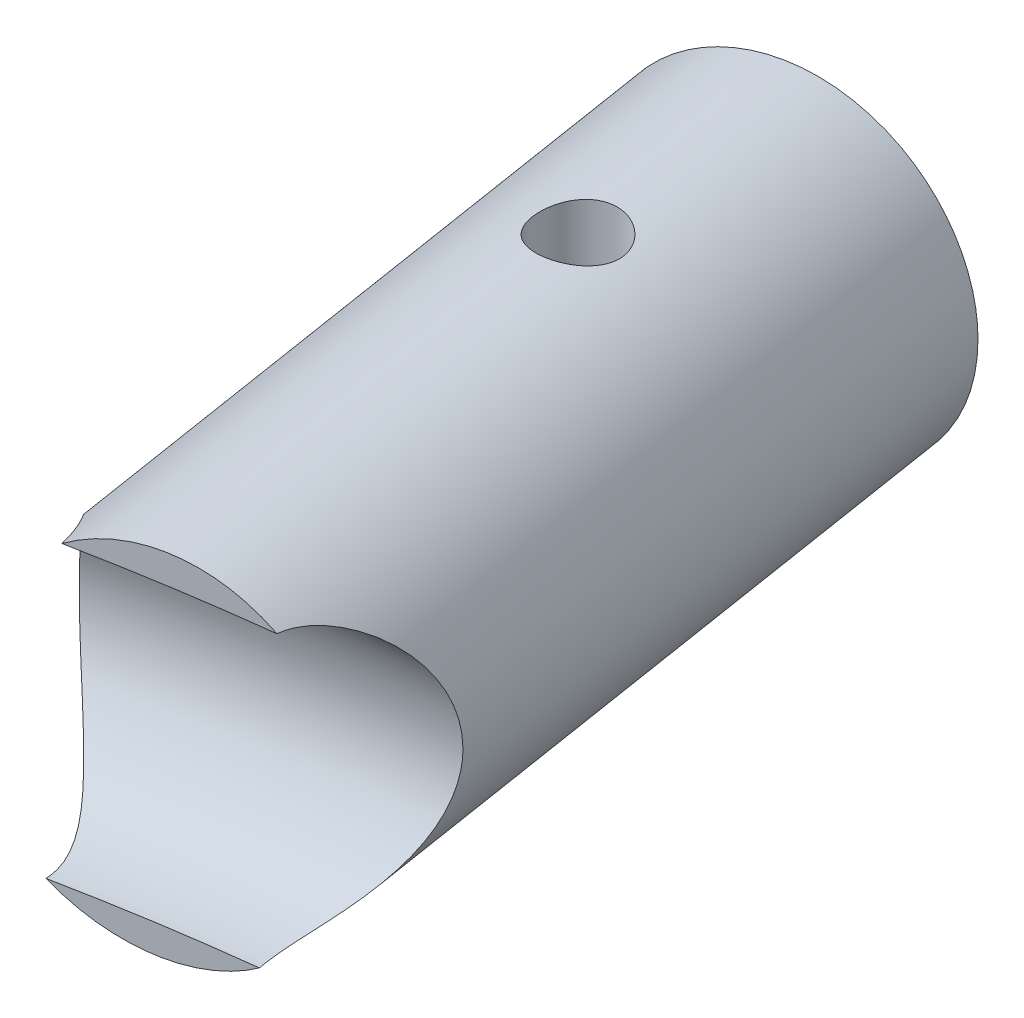
from build123d import *

# Parameters (mm, degrees)
HOLE_SIZE_PER_SOCKET_HEAD_CAP_SCREW_TYPE_D           = 18
HOLE_SIZE_PER_SOCKET_HEAD_CAP_SCREW_TYPE_CBORE_D     = 26
HOLE_SIZE_PER_SOCKET_HEAD_CAP_SCREW_TYPE_CBORE_DEPTH = 21
CIRPATTERN2_COUNT                                    = 20
SKETCH5_OUTSIDE_W                                    = 667.458
SKETCH5_OUTSIDE_H                                    = 191.296
SKETCH5_OUTSIDE_R                                    = 12.5
CUT_EXTRUDE2_DEPTH                                   = 335.405442539
F_6_0_6_DIAMETER_HOLE1_D                             = 6


with BuildPart() as part:
    # Sketch1 → Revolve1 (revolve)
    with BuildSketch(Plane.XY, mode=Mode.PRIVATE) as revolve1_sk:
        with BuildLine():
            Line((-176, 0), (-233, 0))
            Line((-233, 0), (-233, 46))
            Line((-233, 46), (-196, 46))
            Line((-196, 46), (-196, 47))
            Line((-196, 47), (-194.03, 47))
            Line((-194.03, 47), (-194.03, 51))
            Line((-194.03, 51), (-196, 51))
            Line((-196, 51), (-196, 57))
            Line((-196, 57), (-190.3, 57))
            Line((-190.3, 57), (-190.3, 53.2))
            Line((-190.3, 53.2), (-183, 53.2))
            Line((-183, 53.2), (-183, 57))
            Line((-183, 57), (-179.375644347, 57))
            Line((-179.375644347, 57), (-177.5, 50))
            Line((-177.5, 50), (-177.5, 38.351811436))
            ThreePointArc((-177.5, 38.351811436), (-186.87290572, 27.249782079), (-176, 17.612026184))
            Line((-176, 17.612026184), (-176, 8.5))
            Line((-176, 8.5), (-184, 8.5))
            Line((-184, 8.5), (-184, 4.5))
            Line((-184, 4.5), (-176, 4.5))
            Line((-176, 4.5), (-176, 0))
        make_face()
    revolve(revolve1_sk.sketch.rotate(Axis((0, 33.104458612, 0), (0, 1, 0)), 270), axis=Axis((0, 33.104458612, 0), (0, 1, 0)))

    # Hole size per socket head cap screw type1 (through all)
    with Locations(Plane.XZ):
        with Locations((-214, 0)):
            hole_size_per_socket_head_cap_screw_type = CounterBoreHole(HOLE_SIZE_PER_SOCKET_HEAD_CAP_SCREW_TYPE_D / 2, HOLE_SIZE_PER_SOCKET_HEAD_CAP_SCREW_TYPE_CBORE_D / 2, HOLE_SIZE_PER_SOCKET_HEAD_CAP_SCREW_TYPE_CBORE_DEPTH)

    # CirPattern2: Hole size per socket head cap screw type1 ×20 about axis
    cirpattern2_axis = Axis((0, 0, 0), (0, 1, 0))
    for i in range(1, CIRPATTERN2_COUNT):
        add(hole_size_per_socket_head_cap_screw_type.rotate(cirpattern2_axis, i * 360 / CIRPATTERN2_COUNT), mode=Mode.SUBTRACT)

    # Sketch5 outside → Cut-Extrude2 (cut, through all)
    with BuildSketch(Plane(origin=(0, 0, 0), x_dir=(-0.9876883405951378, 0, 0.15643446504023129), z_dir=(-0.15643446504023129, 0, -0.9876883405951378))):
        with Locations((0, 28.5)):
            Rectangle(SKETCH5_OUTSIDE_W, SKETCH5_OUTSIDE_H)
        with Locations(Location((0, 28, 0), (0, 0, 180))):
            Circle(SKETCH5_OUTSIDE_R, mode=Mode.SUBTRACT)
    extrude(amount=CUT_EXTRUDE2_DEPTH, mode=Mode.SUBTRACT)


with BuildPart() as body_2:
    # of the pieces the cut leaves, the one that is kept (cut_extrude2_keep)
    add(part.part.solids().sort_by_distance((-20.643876308, 17.612026184, -174.78509768))[0])

    # Ø6.0 (6) Diameter Hole1 (through all)
    with Locations(Plane(origin=(-33.476975519, 40.5, -211.365304887), x_dir=(0, 0, 1), z_dir=(0, 1, 0))):
        with Locations((0, 0)):
            Hole(F_6_0_6_DIAMETER_HOLE1_D / 2)


solid = body_2.part
